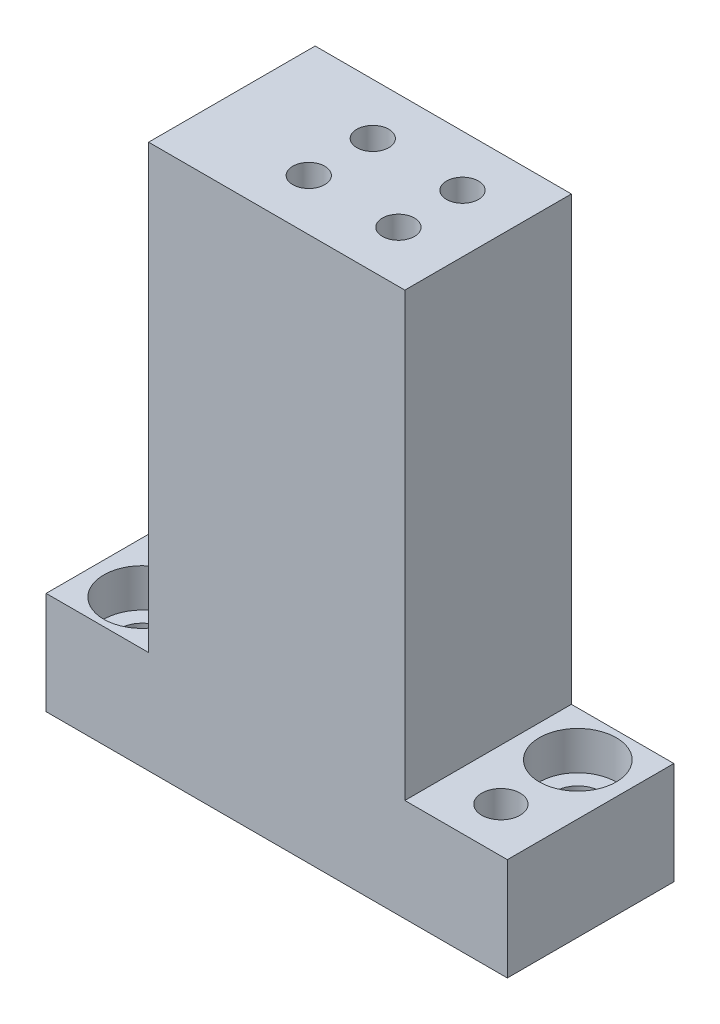
from build123d import *

# Parameters (mm, degrees)
SKETCH1_W           = 72
SKETCH1_H           = 26
BOSS_EXTRUDE1_DEPTH = 16
SKETCH2_W           = 40
SKETCH2_H           = 26
BOSS_EXTRUDE2_DEPTH = 69
SKETCH3_R           = 3.5
SKETCH3_R_2         = 3
CUT_EXTRUDE1_DEPTH  = 96.5
SKETCH4_R           = 6
CUT_EXTRUDE2_DEPTH  = 6
SKETCH5_R           = 2.5
CUT_EXTRUDE3_DEPTH  = 15


with BuildPart() as part:
    # Sketch1 → Boss-Extrude1 (new body)
    with BuildSketch(Plane(origin=(0, 0, 0), x_dir=(1, 0, 0), z_dir=(0, 1, 0))):
        Rectangle(SKETCH1_W, SKETCH1_H)
    extrude(amount=BOSS_EXTRUDE1_DEPTH)

    # Sketch2 → Boss-Extrude2 (add)
    with BuildSketch(Plane(origin=(0, 16, 0), x_dir=(1, 0, 0), z_dir=(0, 1, 0))):
        Rectangle(SKETCH2_W, SKETCH2_H)
    extrude(amount=BOSS_EXTRUDE2_DEPTH)

    # Sketch3 → Cut-Extrude1 (cut)
    with BuildSketch(Plane(origin=(0, 16, 0), x_dir=(1, 0, 0), z_dir=(0, 1, 0))):
        with Locations(Location((28, 6, 0), (0, 0, 270))):
            Circle(SKETCH3_R)
        with Locations(Location((28, -6, 0), (0, 0, 270))):
            Circle(SKETCH3_R_2)
        with Locations(Location((-28, -6, 0), (0, 0, 270))):
            Circle(SKETCH3_R)
        with Locations(Location((-28, 6, 0), (0, 0, 270))):
            Circle(SKETCH3_R_2)
    extrude(amount=-CUT_EXTRUDE1_DEPTH, mode=Mode.SUBTRACT)

    # Sketch4 → Cut-Extrude2 (cut)
    with BuildSketch(Plane(origin=(0, 16, 0), x_dir=(1, 0, 0), z_dir=(0, 1, 0))):
        with Locations(Location((28, 6, 0), (0, 0, 270))):
            Circle(SKETCH4_R)
        with Locations(Location((-28, -6, 0), (0, 0, 270))):
            Circle(SKETCH4_R)
    extrude(amount=-CUT_EXTRUDE2_DEPTH, mode=Mode.SUBTRACT)

    # Sketch5 → Cut-Extrude3 (cut)
    with BuildSketch(Plane(origin=(0, 85, 0), x_dir=(1, 0, 0), z_dir=(0, 1, 0))):
        with Locations(Location((-3, 5, 0), (0, 0, 270))):
            Circle(SKETCH5_R)
        with Locations(Location((11, 5, 0), (0, 0, 270))):
            Circle(SKETCH5_R)
        with Locations(Location((11, -5, 0), (0, 0, 270))):
            Circle(SKETCH5_R)
        with Locations(Location((-3, -5, 0), (0, 0, 270))):
            Circle(SKETCH5_R)
    extrude(amount=-CUT_EXTRUDE3_DEPTH, mode=Mode.SUBTRACT)


solid = part.part
